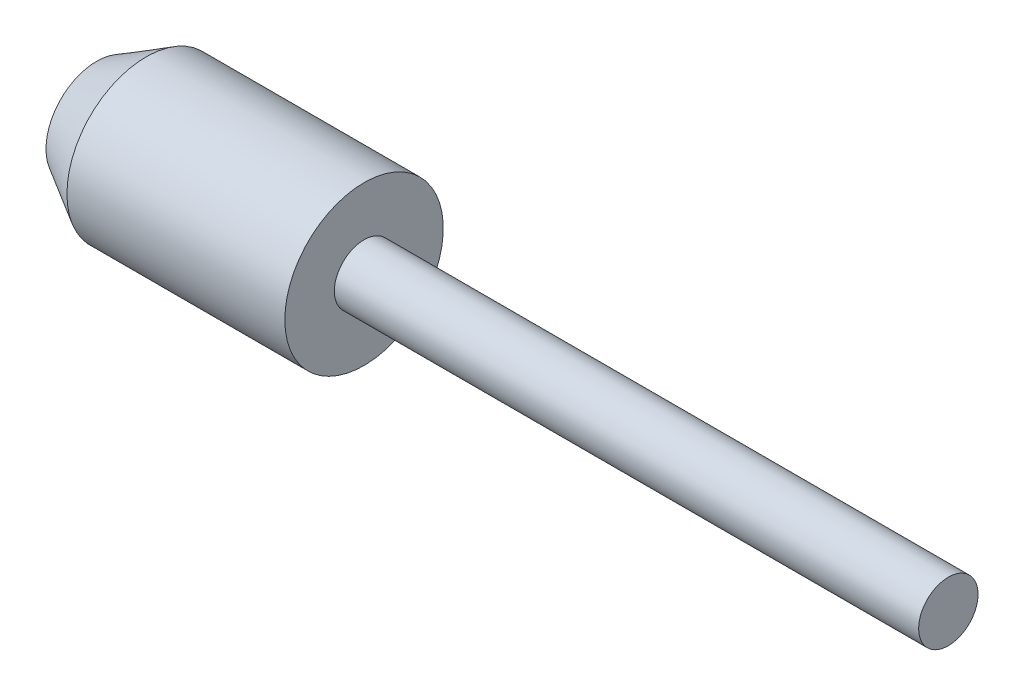
SolidWorks part; units mm, degrees
material "S45C"
ref_plane "Front Plane" through (0, 0, 0) normal (0, 0, 1) x (1, 0, 0)
ref_plane "Top Plane" through (0, 0, 0) normal (0, 1, 0) x (1, 0, 0)
ref_plane "Right Plane" through (0, 0, 0) normal (1, 0, 0) x (0, 0, -1)
sketch "Sketch1" plane through (0, 0, 0) normal (0, 0, 1) x (1, 0, 0)
  line L0 (0, 0) -> (147.2098, 0) construction
  line L1 (0, 0) -> (0, 5.1132)
  line L2 (0, 5.1132) -> (5, 8)
  line L3 (5, 8) -> (27, 8)
  line L4 (27, 8) -> (27, 3)
  line L5 (27, 3) -> (86, 3)
  line L6 (86, 3) -> (86, 0)
  line L7 (0, 0) -> (86, 0)
  dimension "D1" = 16
  dimension "D2" = 6
  dimension "D3" = 5
  dimension "D4" = 30
  dimension "D5" = 27
  dimension "D6" = 59
revolve "Revolve1" add sketch "Sketch1" angle 360 about L0
